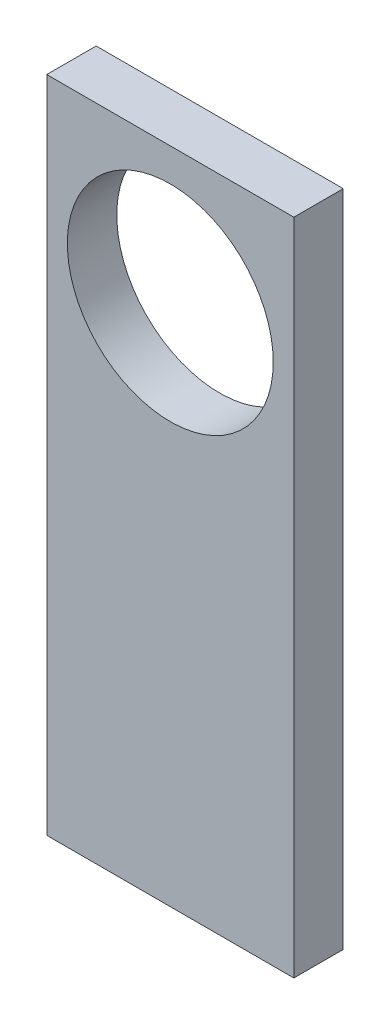
SolidWorks part; units mm, degrees
ref_plane "前视基准面" through (0, 0, 0) normal (0, 0, 1) x (1, 0, 0)
ref_plane "上视基准面" through (0, 0, 0) normal (0, 1, 0) x (1, 0, 0)
ref_plane "右视基准面" through (0, 0, 0) normal (1, 0, 0) x (0, 0, -1)
sketch "草图1" plane through (0, 0, 0) normal (0, 0, 1) x (1, 0, 0)
  line L1 (-30, -80) -> (30, -80)
  line L2 (-30, -80) -> (-30, 80)
  line L3 (-30, 80) -> (30, 80)
  line L4 (30, -80) -> (30, 80)
  line L5 (-30, -80) -> (30, 80) construction
  line L6 (-30, 80) -> (30, -80) construction
  point P0 (0, 0)
  dimension "D1" = 60
  dimension "D2" = 160
extrude "凸台-拉伸1" add sketch "草图1" along normal blind 12
sketch "草图2" plane through (0, 0, 12) normal (0, 0, 1) x (1, 0, 0)
  line L0 (0, 0) -> (0, 80) construction
  line L1 (30, 80) -> (-30, 80) construction
  line L2 (-30, -80) -> (30, -80) construction
  circle A0 centre (0, 47) radius 25
  dimension "D1" = 50
  dimension "D2" = 127
extrude "切除-拉伸1" cut sketch "草图2" against normal through all
